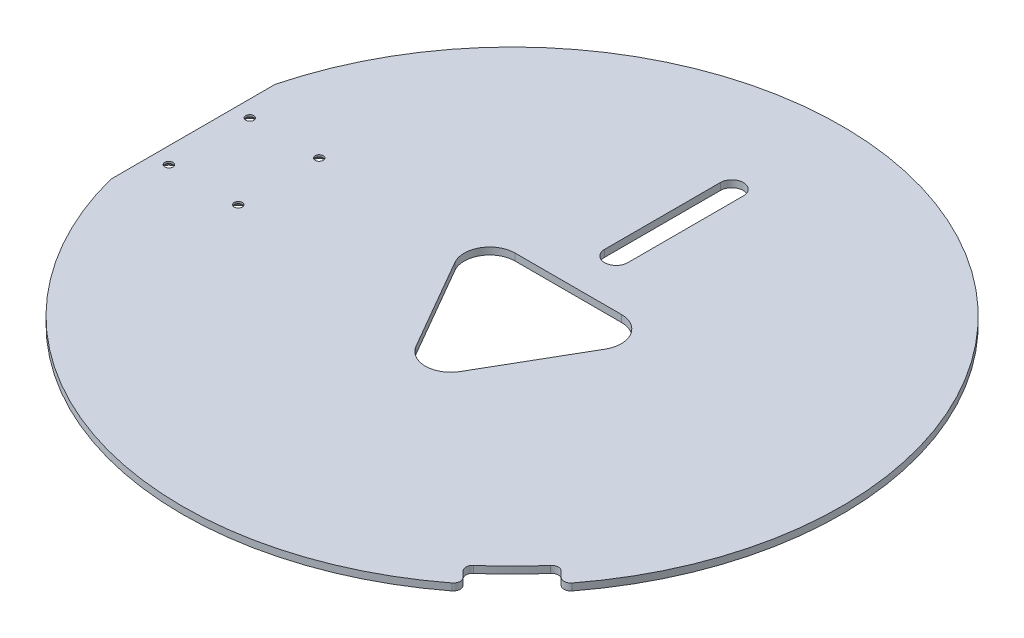
SolidWorks part; units mm, degrees
ref_plane "Front Plane" through (0, 0, 0) normal (0, 0, 1) x (1, 0, 0)
ref_plane "Top Plane" through (0, 0, 0) normal (0, 1, 0) x (1, 0, 0)
ref_plane "Right Plane" through (0, 0, 0) normal (1, 0, 0) x (0, 0, -1)
sketch "Sketch1" plane through (0, 0, 0) normal (0, 1, 0) x (1, 0, 0)
  circle A0 centre (0, 0) radius 142.5
  dimension "D1" = 285
extrude "Boss-Extrude1" add sketch "Sketch1" along normal blind 3
sketch "Sketch3" plane through (0, 3, 0) normal (0, 1, 0) x (1, 0, 0)
  line L0 (0, 0) -> (0, -50000) construction
  circle A0 centre (0, 0) radius 35 construction
  circle A1 centre (0, -26.5) radius 8.5 construction
  circle A2 centre (0, -26.5) radius 11
  dimension "D1" = 70
  dimension "D2" = 17
  dimension "D3" = 22
extrude "Cut-Extrude1" cut sketch "Sketch3" against normal blind 10
pattern_circular "CirPattern1" count 3 over 360 about axis through (0, 0, 0) along (0, 1, 0) of "Cut-Extrude1"
sketch "Sketch4" plane through (0, 3, 0) normal (0, 1, 0) x (1, 0, 0)
  line L0 (-32.476, 7.75) -> (-9.5263, -32)
  line L1 (-22.9497, 24.25) -> (22.9497, 24.25)
  line L2 (32.476, 7.75) -> (9.5263, -32)
  circle A3 centre (-22.9497, 13.25) radius 11 construction
  circle A5 centre (22.9497, 13.25) radius 11 construction
  circle A6 centre (0, -26.5) radius 11 construction
  arc A7 (-22.9497, 24.25) -> (-32.476, 7.75) centre (-22.9497, 13.25) ccw
  arc A8 (32.476, 7.75) -> (22.9497, 24.25) centre (22.9497, 13.25) ccw
  arc A9 (-9.5263, -32) -> (9.5263, -32) centre (0, -26.5) ccw
extrude "Cut-Extrude2" cut sketch "Sketch4" against normal blind 10
sketch "Sketch5" plane through (0, 3, 0) normal (0, 1, 0) x (1, 0, 0)
  line L0 (0, 0) -> (0, 50000) construction
  line L1 (0, 45) -> (0, 95) construction
  line L2 (-5, 45) -> (-5, 95)
  line L3 (5, 45) -> (5, 95)
  line L4 (0, 0) -> (50000, 0) construction
  arc A0 (-5, 45) -> (5, 45) centre (0, 45) ccw
  arc A1 (5, 95) -> (-5, 95) centre (0, 95) ccw
  point P5 (0, 70)
  dimension "D1" = 45
  dimension "D2" = 50
  dimension "D3" = 10
extrude "Cut-Extrude3" cut sketch "Sketch5" against normal blind 10
sketch "Sketch6" plane through (0, 3, 0) normal (0, 1, 0) x (1, 0, 0)
  line L0 (0, 0) -> (50000, 0) construction
  line L1 (0, 0) -> (0, -50000) construction
  line L2 (0, 0) -> (35355.3391, -35355.3391) construction
  line L3 (89.5963, -110.8095) -> (82.4827, -103.6959)
  line L4 (110.8095, -89.5963) -> (103.6959, -82.4827)
  arc A0 (82.4827, -103.6959) -> (103.6959, -82.4827) centre (0, 0) ccw construction
  arc A1 (82.4827, -103.6959) -> (103.6959, -82.4827) centre (0, 0) ccw
  circle A2 centre (0, 0) radius 142.5 construction
  arc A3 (89.5963, -110.8095) -> (110.8095, -89.5963) centre (0, 0) ccw
  dimension "D2" = 265
  dimension "D1" = 45
  dimension "D3" = 30
extrude "Cut-Extrude6" cut sketch "Sketch6" against normal blind 10
fillet "Fillet1" radius 3 4 edges at (103.6959, 1.5, 82.4827) (82.4827, 1.5, 103.6959) (89.5963, 1.5, 110.8095) (110.8095, 1.5, 89.5963)
sketch "Sketch7" plane through (0, 3, 0) normal (0, 1, 0) x (1, 0, 0)
  line L0 (0, 0) -> (50000, 0) construction
  line L2 (-147, 60) -> (-138, 60)
  line L3 (-147, 60) -> (-147, -60)
  line L4 (-147, -60) -> (-138, -60)
  line L5 (-138, 60) -> (-138, -60)
  line L6 (-147, 60) -> (-138, -60) construction
  line L7 (-147, -60) -> (-138, 60) construction
  arc A0 (112.922, -86.9187) -> (86.9187, -112.922) centre (0, 0) ccw construction
  point P3 (-142.5, 0)
  dimension "D1" = 138
  dimension "D2" = 120
extrude "Cut-Extrude7" cut sketch "Sketch7" against normal blind 10
sketch "Sketch8" plane through (0, 3, 0) normal (0, 1, 0) x (1, 0, 0)
  line L0 (0, 0) -> (-50000, 0) construction
  circle A0 centre (-130.8924, 17.5) radius 1.75
  circle A1 centre (-100.8924, 17.5) radius 1.75
  circle A2 centre (-130.8924, -17.5) radius 1.75
  circle A3 centre (-100.8924, -17.5) radius 1.75
  dimension "D1" = 3.5
  dimension "D2" = 30
  dimension "D3" = 35
  dimension "D4" = 100.8924
extrude "Cut-Extrude8" cut sketch "Sketch8" against normal blind 10
chamfer "Chamfer1" distance 2.2 angle 45 4 edges at (-130.8924, 0, 19.25) (-100.8924, 0, 19.25) (-130.8924, 0, -15.75) (-100.8924, 0, -15.75)
